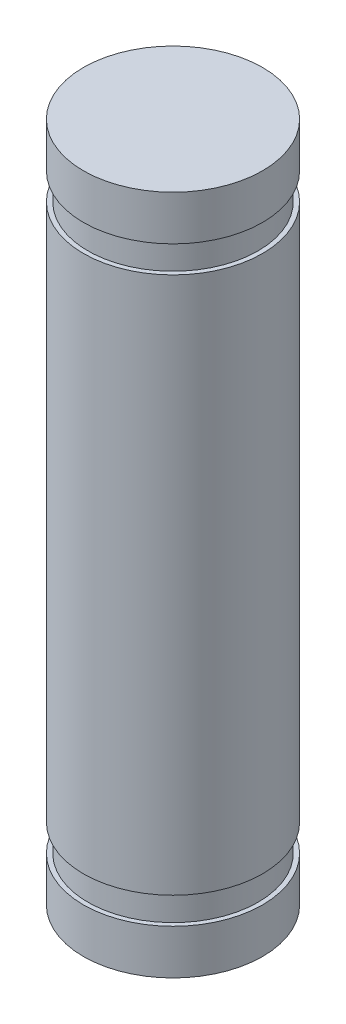
from build123d import *


with BuildPart() as part:
    # 草图1 → 旋转1 (revolve)
    with BuildSketch(Plane.XY, mode=Mode.PRIVATE) as revolve_1_sk:
        Polygon((0, 2.646643634), (2, 2.646643634), (2, 1.646643634), (1.9, 1.646643634), (1.9, 1.046643634), (2, 1.046643634), (2, -10.953356366), (1.9, -10.953356366), (1.9, -11.553356366), (2, -11.553356366), (2, -12.553356366), (0, -12.553356366), align=None)
    revolve(revolve_1_sk.sketch.rotate(Axis((0, 2.646643634, 0), (0, -1, 0)), 180), axis=Axis((0, 2.646643634, 0), (0, -1, 0)))


solid = part.part
